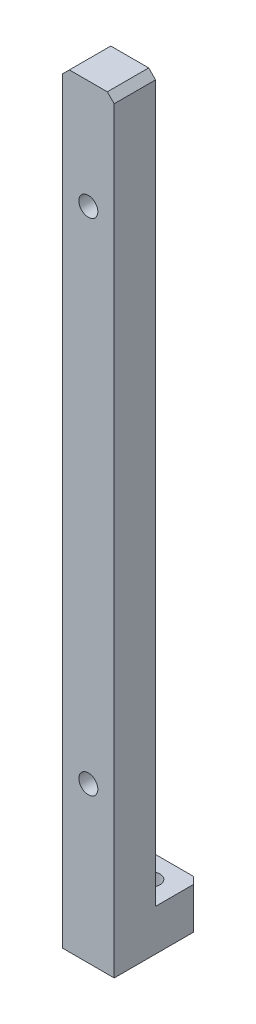
SolidWorks part; units mm, degrees
material "A6061"
ref_plane "Front Plane" through (0, 0, 0) normal (0, 0, 1) x (1, 0, 0)
ref_plane "Top Plane" through (0, 0, 0) normal (0, 1, 0) x (1, 0, 0)
ref_plane "Right Plane" through (0, 0, 0) normal (1, 0, 0) x (0, 0, -1)
sketch "Sketch1" plane through (0, 0, 0) normal (1, 0, 0) x (0, 0, -1)
  line L0 (0, 0) -> (25, 0)
  line L1 (25, 0) -> (25, 12)
  line L2 (25, 12) -> (12, 12)
  line L3 (12, 12) -> (12, 221.5)
  line L4 (12, 221.5) -> (0, 221.5)
  line L5 (0, 221.5) -> (0, 0)
  dimension "D1" = 25
  dimension "D2" = 12
  dimension "D3" = 12
  dimension "D4" = 221.5
extrude "Boss-Extrude1" add sketch "Sketch1" along normal blind 15
hole_wizard "CBORE for M5 Hexagon socket head cap screws1" positions "Sketch2" profile "Sketch3" counterbore size "M5" standard "GB" end condition through all
sketch "Sketch2" plane through (0, 0, -12) normal (0, 0, -1) x (-1, 0, 0)
  line L0 (-7.5, 221.5) -> (-7.5, 0) construction
  line L1 (-15, 221.5) -> (0, 221.5) construction
  line L2 (-15, 0) -> (0, 0) construction
  point P9 (-7.5, 190)
  point P11 (-7.5, 45)
  dimension "D1" = 45
  dimension "D2" = 145
sketch "Sketch3" plane through (7.5, 45, -12) normal (1, 0, 0) x (0, 1, 0)
  line L0 (0, 0) -> (0, 12)
  line L1 (0, 12) -> (2.75, 12)
  line L3 (2.75, 12) -> (2.75, 5.7)
  line L4 (2.75, 5.7) -> (5, 5.7)
  line L5 (5, 5.7) -> (5, 0)
  line L7 (5, 0) -> (0, 0)
  line L11 (0, -6.35) -> (0, 107.95) construction
  dimension "通孔孔直径" = 5.5
  dimension "通孔孔深度" = 12
  dimension "柱形沉头孔直径" = 10
  dimension "柱形沉头孔深度" = 5.7
hole_wizard "M5 Clearance Hole1" positions "Sketch4" profile "Sketch5" hole size "M5" standard "GB" end condition through all
sketch "Sketch4" plane through (0, 0, 0) normal (0, -1, 0) x (-1, 0, 0)
  line L0 (-7.5, 25) -> (-7.5, 0) construction
  line L1 (-15, 25) -> (0, 25) construction
  line L2 (-15, 0) -> (0, 0) construction
  point P9 (-7.5, 18)
  dimension "D1" = 18
sketch "Sketch5" plane through (7.5, 0, -18) normal (1, 0, 0) x (0, 0, -1)
  line L0 (0, 0) -> (0, 221.5)
  line L1 (0, 221.5) -> (2.75, 221.5)
  line L2 (2.75, 221.5) -> (2.75, 0)
  line L5 (2.75, 0) -> (0, 0)
  line L11 (0, -6.35) -> (0, 107.95) construction
  dimension "通孔孔直径" = 5.5
  dimension "通孔孔深度" = 221.5
chamfer "Chamfer1" distance 2 angle 45 4 edges at (0, 6, -25) (15, 6, -25) (0, 221.5, -6) (15, 221.5, -6)
